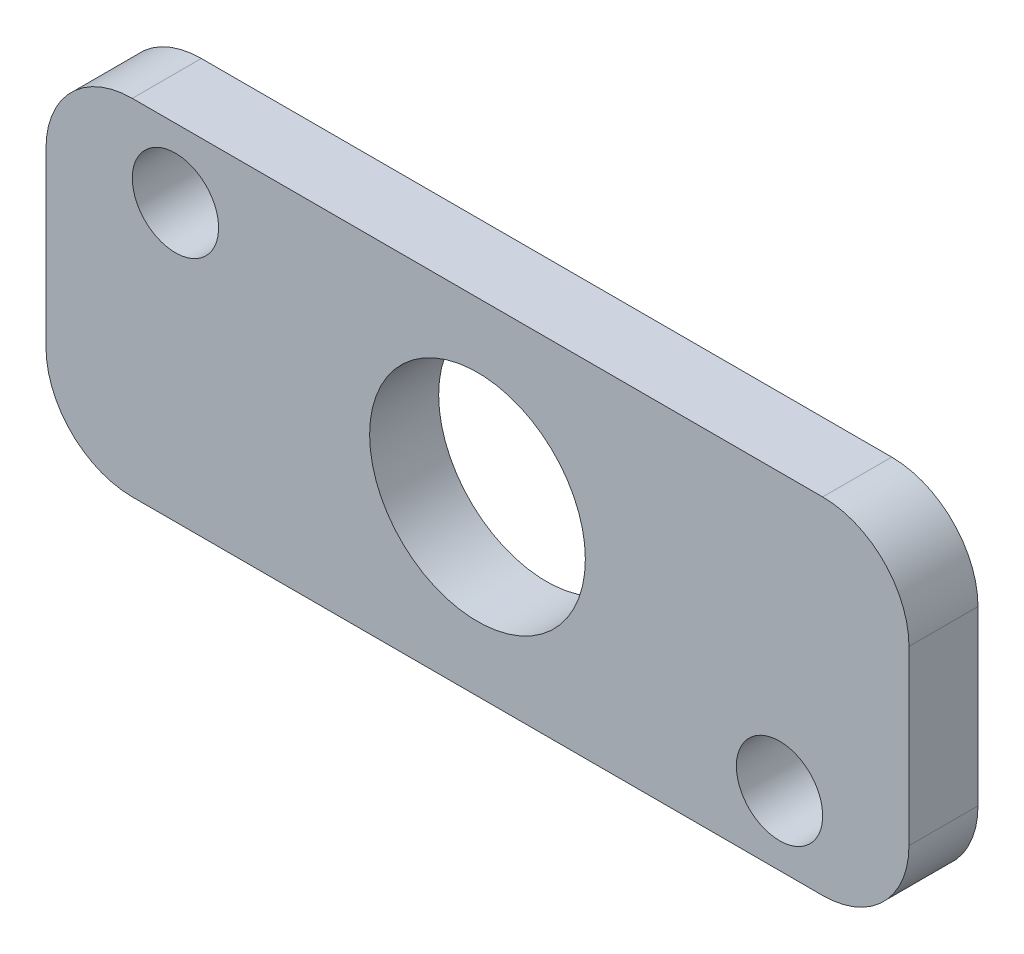
SolidWorks part; units mm, degrees
material "1023 碳钢板 (SS)"
ref_plane "前视基准面" through (0, 0, 0) normal (0, 0, 1) x (1, 0, 0)
ref_plane "上视基准面" through (0, 0, 0) normal (0, 1, 0) x (1, 0, 0)
ref_plane "右视基准面" through (0, 0, 0) normal (1, 0, 0) x (0, 0, -1)
ref_plane "基准面4" through (0, 0, 2) normal (0, 0, 1) x (1, 0, 0)
sketch "草图1" plane through (0, 0, 2) normal (0, 0, 1) x (1, 0, 0)
  line L0 (-20, -10) -> (20, -10)
  line L1 (25, -5) -> (25, 5)
  line L2 (20, 10) -> (-20, 10)
  line L3 (-25, 5) -> (-25, -5)
  circle A0 centre (-17.5, 6) radius 2.5
  circle A1 centre (17.5, -6) radius 2.5
  circle A2 centre (0, 0) radius 6.25
  arc A3 (20, -10) -> (25, -5) centre (20, -5) ccw
  arc A4 (25, 5) -> (20, 10) centre (20, 5) ccw
  arc A5 (-20, 10) -> (-25, 5) centre (-20, 5) ccw
  arc A6 (-25, -5) -> (-20, -10) centre (-20, -5) ccw
extrude "凸台-拉伸1" add sketch "草图1" against normal blind 4
